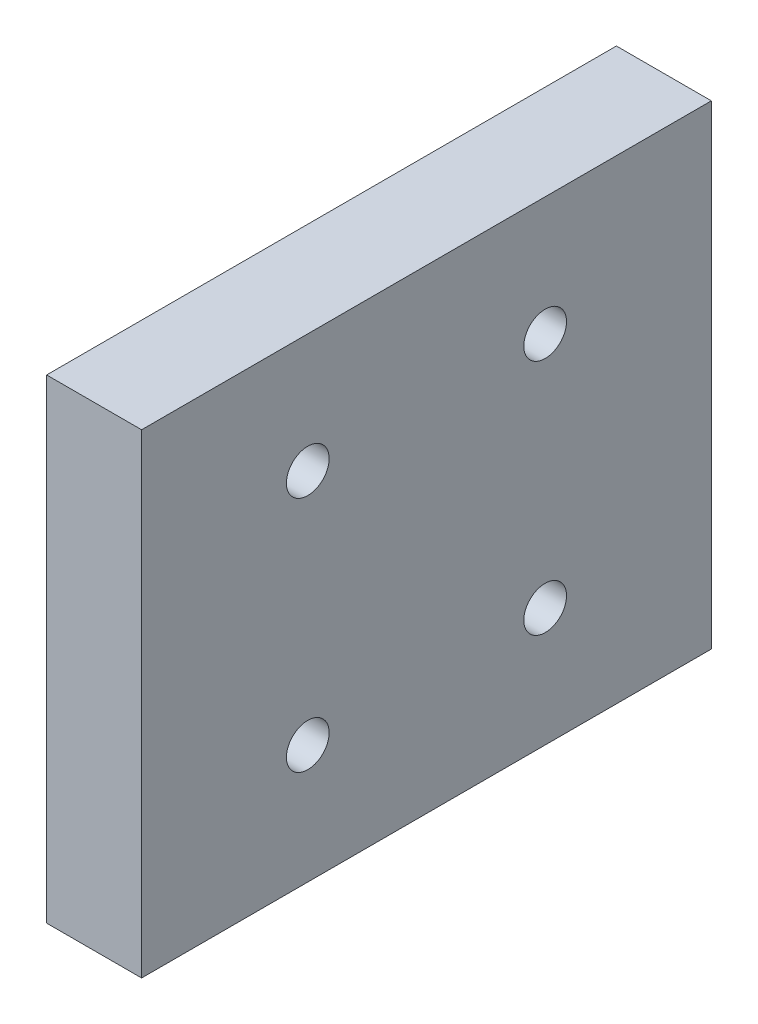
from build123d import *

# Parameters (mm, degrees)
SKETCH_1_W            = 120
SKETCH_1_H            = 100
EXTRUDE_1_DEPTH       = 20
HOLE_WIZARD_9_0_9_1_D = 9


with BuildPart() as part:
    # 草图1 → 凸台-拉伸1 (new body)
    with BuildSketch(Plane(origin=(0, 0, 0), x_dir=(0, 0, -1), z_dir=(1, 0, 0))):
        Rectangle(SKETCH_1_W, SKETCH_1_H)
    extrude(amount=EXTRUDE_1_DEPTH)

    # Ø9.0 (9) 直径孔1 (through all)
    with Locations(Plane(origin=(20, 0, 0), x_dir=(0, 0, -1), z_dir=(1, 0, 0))):
        with Locations((-25, 25), (25, 25), (-25, -25), (25, -25)):
            Hole(HOLE_WIZARD_9_0_9_1_D / 2)


solid = part.part
